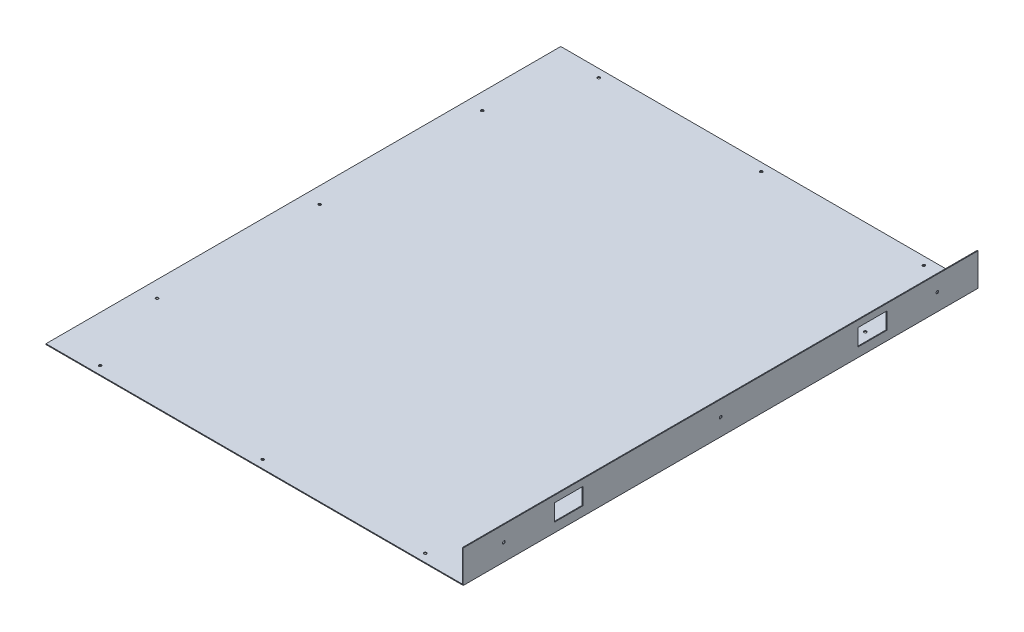
from build123d import *

# Parameters (mm, degrees)
BOSS_EXTRUDE1_DEPTH = 950
SKETCH2_R           = 2.5
SKETCH2_W           = 53
SKETCH2_H           = 31
CUT_EXTRUDE1_DEPTH  = 1356.5
SKETCH3_R           = 2.5
CUT_EXTRUDE2_DEPTH  = 1.5
SKETCH4_W           = 1.5
SKETCH4_H           = 950
CUT_EXTRUDE3_DEPTH  = 58.5


with BuildPart() as part:
    # Sketch1 → Boss-Extrude1 (new body)
    with BuildSketch(Plane.XY):
        Polygon((0, 0), (0, -60), (770, -60), (770, 0), (768.5, 0), (768.5, -58.5), (1.5, -58.5), (1.5, 0), align=None)
    extrude(amount=BOSS_EXTRUDE1_DEPTH)

    # Sketch2 → Cut-Extrude1 (cut)
    with BuildSketch(Plane(origin=(770, 0, 0), x_dir=(0, 0, -1), z_dir=(1, 0, 0))):
        with Locations(Location((-75, -28.5, 0), (0, 0, 270))):
            Circle(SKETCH2_R)
        with Locations(Location((-475, -28.5, 0), (0, 0, 270))):
            Circle(SKETCH2_R)
        with Locations(Location((-875, -28.5, 0), (0, 0, 270))):
            Circle(SKETCH2_R)
        with Locations((-194.5, -27.5)):
            Rectangle(SKETCH2_W, SKETCH2_H)
        with Locations((-755.5, -27.5)):
            Rectangle(SKETCH2_W, SKETCH2_H)
    extrude(amount=-CUT_EXTRUDE1_DEPTH, mode=Mode.SUBTRACT)

    # Sketch3 → Cut-Extrude2 (cut)
    with BuildSketch(Plane.XZ.offset(60)):
        with Locations(Location((737, 475, 0), (0, 0, 270))):
            Circle(SKETCH3_R)
        with Locations(Location((737, 775, 0), (0, 0, 270))):
            Circle(SKETCH3_R)
        with Locations(Location((737, 175, 0), (0, 0, 270))):
            Circle(SKETCH3_R)
        with Locations(Location((30, 775, 0), (0, 0, 270))):
            Circle(SKETCH3_R)
        with Locations(Location((30, 475, 0), (0, 0, 270))):
            Circle(SKETCH3_R)
        with Locations(Location((30, 175, 0), (0, 0, 270))):
            Circle(SKETCH3_R)
        with Locations(Location((385, 935, 0), (0, 0, 270))):
            Circle(SKETCH3_R)
        with Locations(Location((685, 935, 0), (0, 0, 270))):
            Circle(SKETCH3_R)
        with Locations(Location((85, 935, 0), (0, 0, 270))):
            Circle(SKETCH3_R)
        with Locations(Location((85, 15, 0), (0, 0, 90))):
            Circle(SKETCH3_R)
        with Locations(Location((685, 15, 0), (0, 0, 90))):
            Circle(SKETCH3_R)
        with Locations(Location((385, 15, 0), (0, 0, 90))):
            Circle(SKETCH3_R)
    extrude(amount=-CUT_EXTRUDE2_DEPTH, mode=Mode.SUBTRACT)

    # Sketch4 → Cut-Extrude3 (cut)
    with BuildSketch(Plane(origin=(0, 0, 0), x_dir=(1, 0, 0), z_dir=(0, 1, 0))):
        with Locations((0.75, -475)):
            Rectangle(SKETCH4_W, SKETCH4_H)
    extrude(amount=-CUT_EXTRUDE3_DEPTH, mode=Mode.SUBTRACT)


solid = part.part
